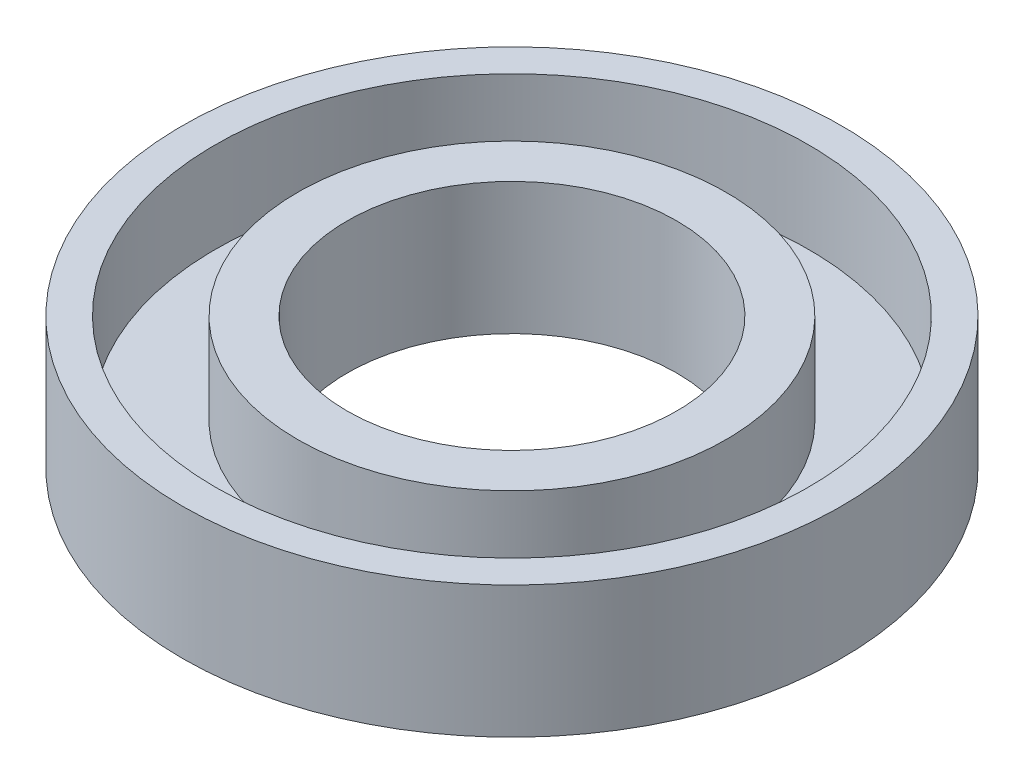
SolidWorks part; units mm, degrees
ref_plane "Front Plane" through (0, 0, 0) normal (0, 0, 1) x (1, 0, 0)
ref_plane "Top Plane" through (0, 0, 0) normal (0, 1, 0) x (1, 0, 0)
ref_plane "Right Plane" through (0, 0, 0) normal (1, 0, 0) x (0, 0, -1)
other "Configuration Table"
sketch "Sketch1" plane through (0, 0, 0) normal (0, 1, 0) x (1, 0, 0)
  circle A0 centre (0, 0) radius 20
  circle A1 centre (0, 0) radius 10
  dimension "D1" = 40
  dimension "D2" = 20
extrude "Boss-Extrude1" add sketch "Sketch1" along normal blind 8
sketch "Sketch2" plane through (0, 8, 0) normal (0, 1, 0) x (1, 0, 0)
  circle A0 centre (0, 0) radius 18
  circle A1 centre (0, 0) radius 20 construction
  circle A2 centre (0, 0) radius 13
  circle A3 centre (0, 0) radius 10 construction
  dimension "D1" = 2
  dimension "D2" = 3
extrude "Cut-Extrude1" cut sketch "Sketch2" against normal offset from surface (5.5 mm away) 2.5 up to face at (0, 0, 20)
